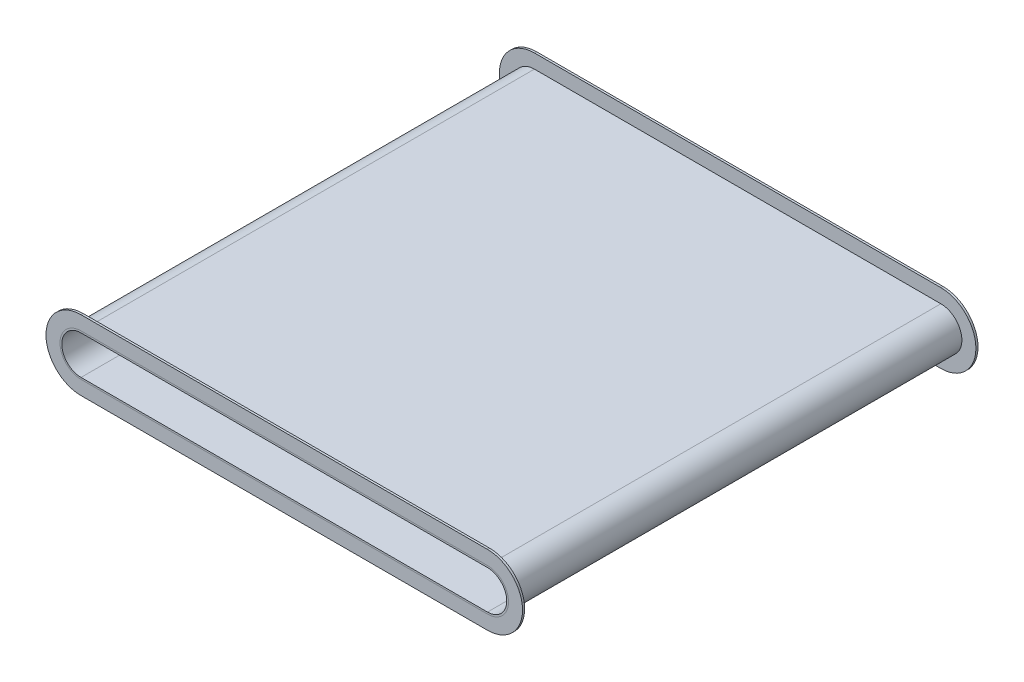
SolidWorks part; units mm, degrees
ref_plane "Front Plane" through (0, 0, 0) normal (0, 0, 1) x (1, 0, 0)
ref_plane "Top Plane" through (0, 0, 0) normal (0, 1, 0) x (1, 0, 0)
ref_plane "Right Plane" through (0, 0, 0) normal (1, 0, 0) x (0, 0, -1)
sketch "Sketch1" plane through (0, 0, 0) normal (0, 0, 1) x (1, 0, 0)
  line L0 (0, 30) -> (580, 30)
  line L1 (0, -30) -> (580, -30)
  line L2 (0, 27.5) -> (580, 27.5)
  line L3 (0, -27.5) -> (580, -27.5)
  arc A0 (0, 30) -> (0, -30) centre (0, 0) ccw
  arc A1 (580, -30) -> (580, 30) centre (580, 0) ccw
  arc A2 (580, -27.5) -> (580, 27.5) centre (580, 0) ccw
  arc A3 (0, 27.5) -> (0, -27.5) centre (0, 0) ccw
  dimension "D2" = 60
  dimension "D1" = 580
  dimension "D3" = 2.5
extrude "Boss-Extrude1" add sketch "Sketch1" along normal mid plane 650
sketch "Sketch2" plane through (0, 0, 325) normal (0, 0, 1) x (1, 0, 0)
  line L0 (580, 50) -> (0, 50)
  line L1 (0, -50) -> (580, -50)
  line L2 (0, -30) -> (580, -30)
  line L3 (580, 30) -> (0, 30)
  line L4 (0, -30) -> (580, -30)
  line L5 (580, 30) -> (0, 30)
  arc A0 (0, 50) -> (0, -50) centre (0, 0) ccw
  arc A1 (580, -50) -> (580, 50) centre (580, 0) ccw
  arc A2 (0, 30) -> (0, -30) centre (0, 0) ccw
  arc A3 (580, -30) -> (580, 30) centre (580, 0) ccw
  arc A4 (0, 30) -> (0, -30) centre (0, 0) ccw
  arc A5 (580, -30) -> (580, 30) centre (580, 0) ccw
  dimension "D1" = 0
  dimension "D2" = 20
extrude "Boss-Extrude2" add sketch "Sketch2" against normal blind 3 separate body
mirror "Mirror1" about plane through (0, 0, 0) normal (0, 0, 1) of bodies 109
